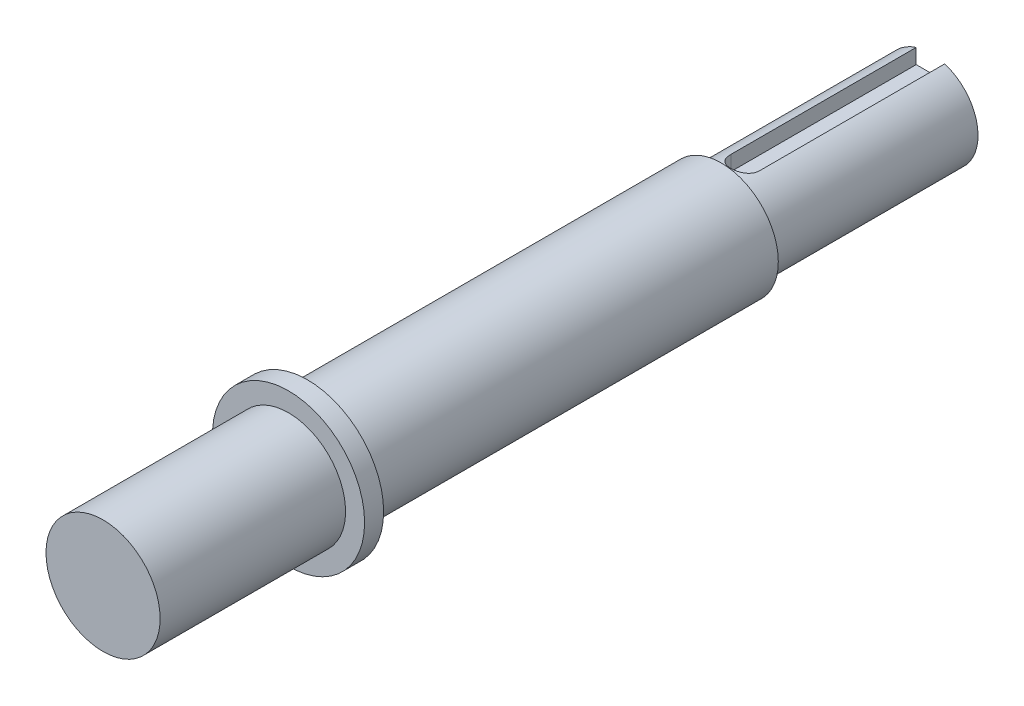
from build123d import *

# Parameters (mm, degrees)
SKETCH_1_R             = 6
EXTRUDE_1_DEPTH        = 65
SKETCH_2_R             = 5
EXTRUDE_2_DEPTH        = 22
SKETCH_3_W             = 2
SKETCH_3_H             = 2
ZJCQC_DEPTH            = 1.8
HOLE_WIZARD_M4_1_D     = 3.3
HOLE_WIZARD_M4_1_DEPTH = 10.1
HOLE_WIZARD_M4_1_TIP   = 0.991420021


with BuildPart() as part:
    # 草图1 → 凸台-拉伸1 (new body)
    with BuildSketch(Plane.XY):
        Circle(SKETCH_1_R)
    extrude(amount=EXTRUDE_1_DEPTH)

    # 草图2 → 凸台-拉伸2 (add)
    with BuildSketch(Plane(origin=(0, 0, 0), x_dir=(-1, 0, 0), z_dir=(0, 0, -1))):
        Circle(SKETCH_2_R)
    extrude(amount=EXTRUDE_2_DEPTH)

    # 草图3 → 旋转1 (revolve)
    with BuildSketch(Plane(origin=(0, 0, 0), x_dir=(1, 0, 0), z_dir=(0, 1, 0)), mode=Mode.PRIVATE) as revolve_1_sk:
        with Locations((-7, -44.5)):
            Rectangle(SKETCH_3_W, SKETCH_3_H)
    revolve(revolve_1_sk.sketch.rotate(Axis((0, 0, 65), (0, 0, -1)), 180), axis=Axis((0, 0, 65), (0, 0, -1)))

    # MyToolsZJC → ZJCQC (cut)
    with BuildSketch(Plane(origin=(0, 5, -22), x_dir=(0, 0, 1), z_dir=(0, 1, 0))):
        with BuildLine():
            Line((-0.5, 1.5), (19.5, 1.5))
            ThreePointArc((19.5, 1.5), (21, 0), (19.5, -1.5))
            Line((19.5, -1.5), (-0.5, -1.5))
            ThreePointArc((-0.5, -1.5), (-2, 0), (-0.5, 1.5))
        make_face()
    extrude(amount=-ZJCQC_DEPTH, mode=Mode.SUBTRACT)

    # M4 螺纹孔1
    with Locations(Plane(origin=(0, 0, -22), x_dir=(-1, 0, 0), z_dir=(0, 0, -1))):
        with Locations((0, 0)):
            Hole(HOLE_WIZARD_M4_1_D / 2, depth=HOLE_WIZARD_M4_1_DEPTH)
            with Locations((0, 0, -(HOLE_WIZARD_M4_1_DEPTH + HOLE_WIZARD_M4_1_TIP / 2))):  # 118° drill point
                Cone(0, HOLE_WIZARD_M4_1_D / 2, HOLE_WIZARD_M4_1_TIP, mode=Mode.SUBTRACT)


solid = part.part
